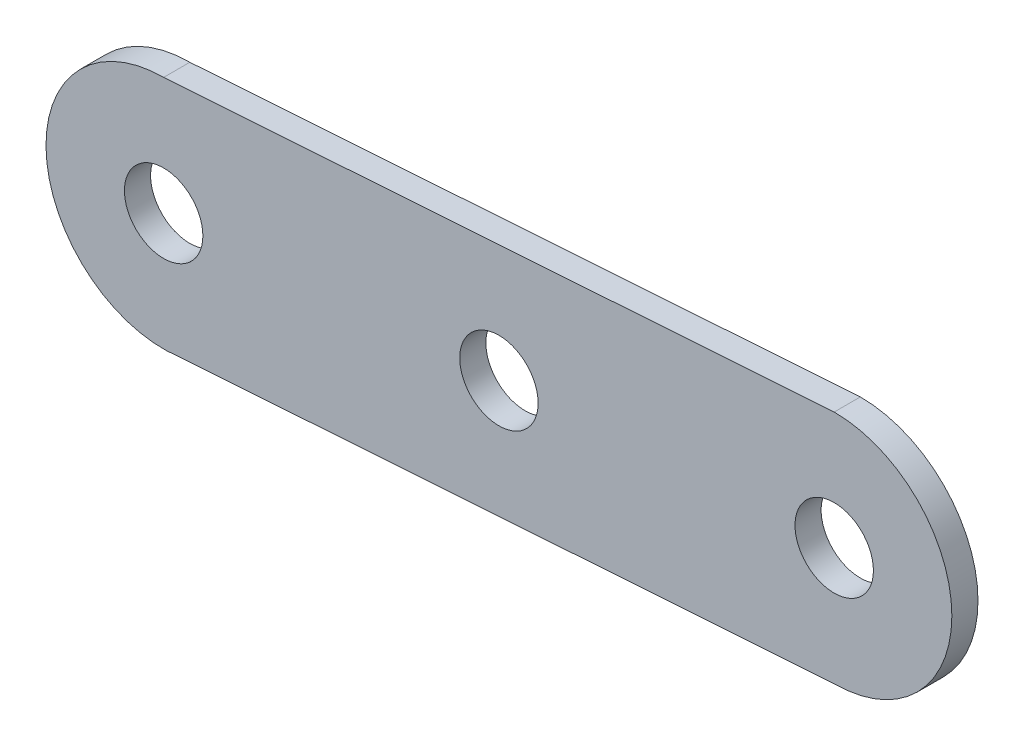
SolidWorks part; units mm, degrees
ref_plane "Front Plane" through (0, 0, 0) normal (0, 0, 1) x (1, 0, 0)
ref_plane "Top Plane" through (0, 0, 0) normal (0, 1, 0) x (1, 0, 0)
ref_plane "Right Plane" through (0, 0, 0) normal (1, 0, 0) x (0, 0, -1)
other "Configuration Table"
sketch "Sketch1" plane through (0, 0, 0) normal (0, 0, 1) x (1, 0, 0)
  line L0 (0, 0) -> (-51.2936, -3.4781) construction
  line L1 (-51.2936, 5.5219) -> (0, 9)
  line L2 (-50.0787, -12.3957) -> (0, -9)
  arc A0 (0, -9) -> (0, 9) centre (0, 0) ccw
  arc A1 (-51.2936, 5.5219) -> (-50.0787, -12.3957) centre (-51.2936, -3.4781) ccw
  circle A2 centre (-51.2936, -3.4781) radius 3
  circle A3 centre (0, 0) radius 3
  circle A4 centre (-25.6468, -1.7391) radius 3
  dimension "D3" = 18
  dimension "D4" = 6
  dimension "D5" = 6
  dimension "D1" = 51.2936
  dimension "D2" = 3.4781
extrude "Boss-Extrude1" add sketch "Sketch1" along normal blind 2
